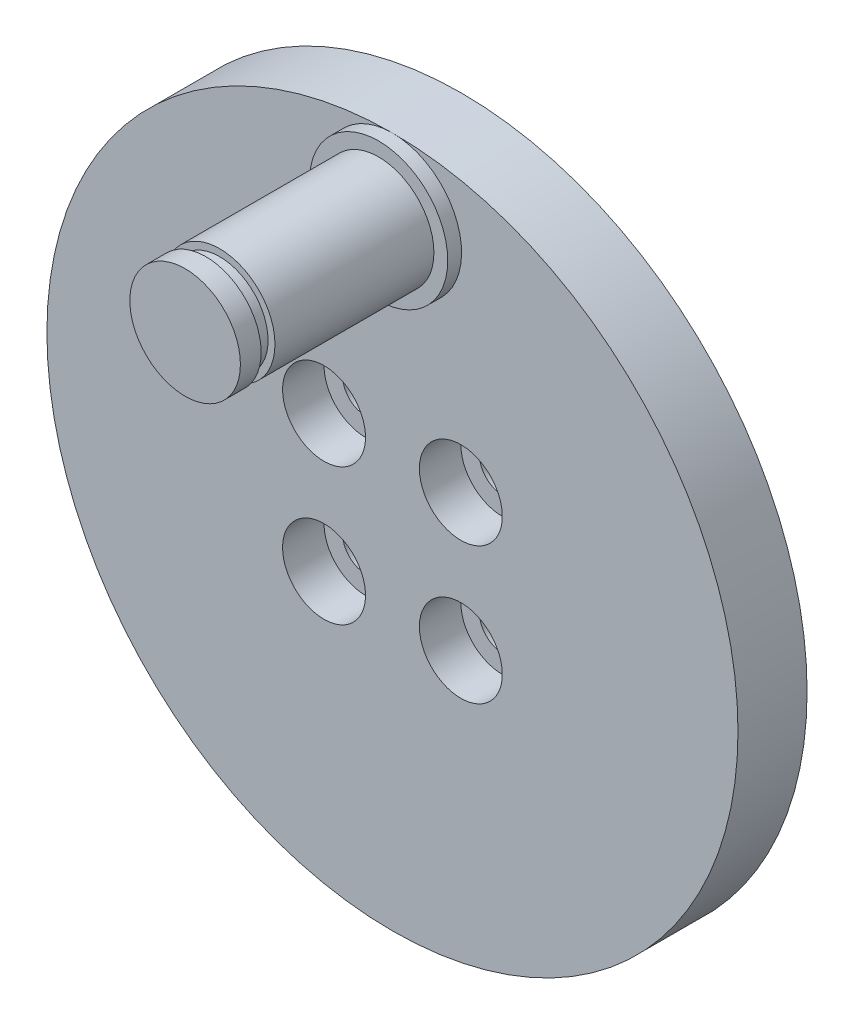
SolidWorks part; units mm, degrees
ref_plane "前视基准面" through (0, 0, 0) normal (0, 0, 1) x (1, 0, 0)
ref_plane "上视基准面" through (0, 0, 0) normal (0, 1, 0) x (1, 0, 0)
ref_plane "右视基准面" through (0, 0, 0) normal (1, 0, 0) x (0, 0, -1)
sketch "草图1" plane through (0, 0, 0) normal (0, 0, 1) x (1, 0, 0)
  circle A0 centre (0, 0) radius 25
  dimension "D1" = 50
extrude "凸台-拉伸1" add sketch "草图1" along normal blind 5
sketch "草图4" plane through (0, 0, 5) normal (0, 0, 1) x (1, 0, 0)
  line L0 (0, 20) -> (0, 0) construction
  line L1 (0, 25) -> (0, 24) construction
  circle A0 centre (0, 20) radius 4
  circle A1 centre (0, 0) radius 25 construction
  dimension "D1" = 8
  dimension "D2" = 1
extrude "凸台-拉伸2" add sketch "草图4" along normal blind 15
sketch "草图6" plane through (0, 0, 0) normal (0, 0, -1) x (-1, 0, 0)
  line L0 (0, 0) -> (0, 13.1032) construction
  line L1 (0, 0) -> (4.9497, 4.9497) construction
  circle A0 centre (4.9497, 4.9497) radius 1.65
  dimension "D2" = 3.3
  dimension "D1" = 45
  dimension "D3" = 7
extrude "切除-拉伸2" cut sketch "草图6" against normal blind 10
pattern_circular "阵列(圆周)1" count 4 over 360 about axis through (0, 0, 0) along (0, 0, 1) of "切除-拉伸2"
sketch "草图7" plane through (0, 0, 5) normal (0, 0, -1) x (-1, 0, 0)
  circle A0 centre (-4.9497, 4.9497) radius 3
  circle A1 centre (4.9497, 4.9497) radius 3
  circle A2 centre (4.9497, -4.9497) radius 3
  circle A3 centre (-4.9497, -4.9497) radius 3
  dimension "D1" = 6
extrude "切除-拉伸3" cut sketch "草图7" along normal blind 3
sketch "草图8" plane through (0, 0, 5) normal (0, 0, 1) x (1, 0, 0)
  circle A0 centre (0, 20) radius 5
  circle A1 centre (0, 20) radius 4 construction
  circle A2 centre (0, 20) radius 4
  dimension "D2" = 1
extrude "凸台-拉伸3" add sketch "草图8" along normal blind 1
sketch "草图10" plane through (0, 0, 20) normal (0, 0, 1) x (1, 0, 0)
  circle A0 centre (0, 20) radius 4
  circle A1 centre (0, 20) radius 4 construction
  circle A2 centre (0, 20) radius 3.5
  dimension "D1" = 0.5
extrude "切除-拉伸4" cut sketch "草图10" against normal blind 1 from offset 1.5
